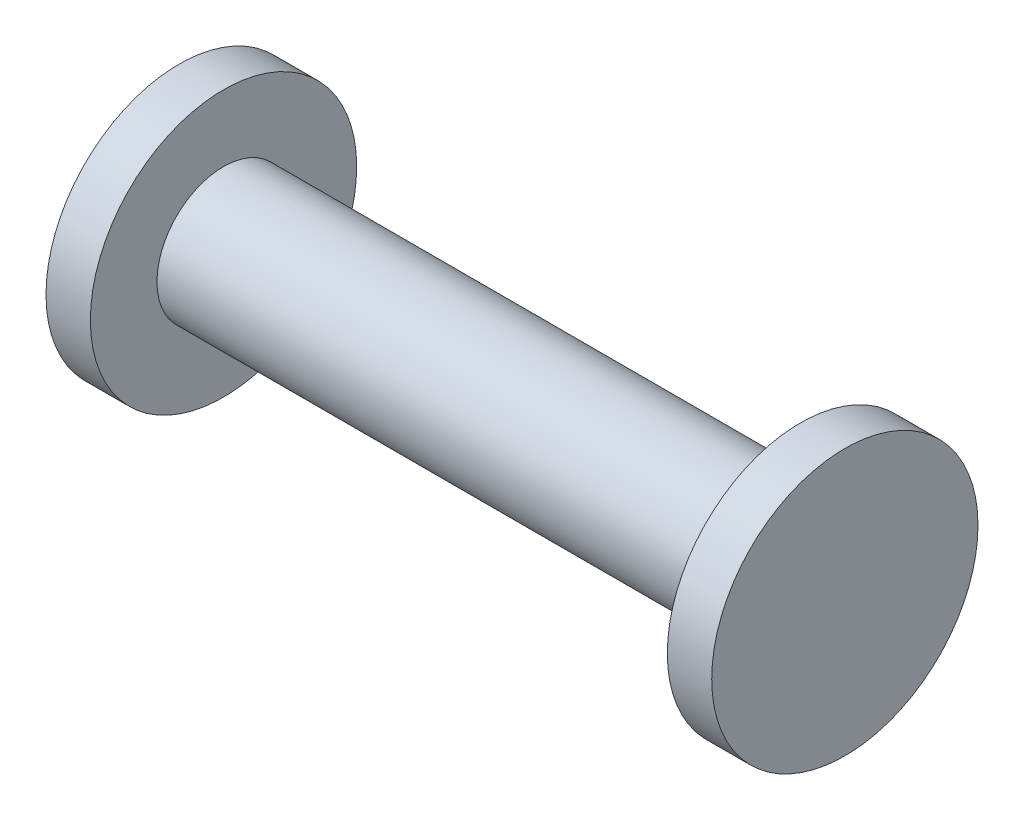
from build123d import *

# Parameters (mm, degrees)
SCALE1_SCALE = 0.3


with BuildPart() as part:
    # Sketch3 → Revolve1 (revolve)
    with BuildSketch(Plane.XY, mode=Mode.PRIVATE) as revolve1_sk:
        Polygon((-37.5, 0), (37.5, 0), (37.5, 15), (32.5, 15), (32.5, 7.5), (-32.5, 7.5), (-32.5, 15), (-37.5, 15), align=None)
    revolve(revolve1_sk.sketch.rotate(Axis((-37.5, 0, 0), (1, 0, 0)), 90), axis=Axis((-37.5, 0, 0), (1, 0, 0)))


with BuildPart() as part_1:
    # Scale1: scaled about (0, 0, 0)
    add(part.part.scale(SCALE1_SCALE))


solid = part_1.part
